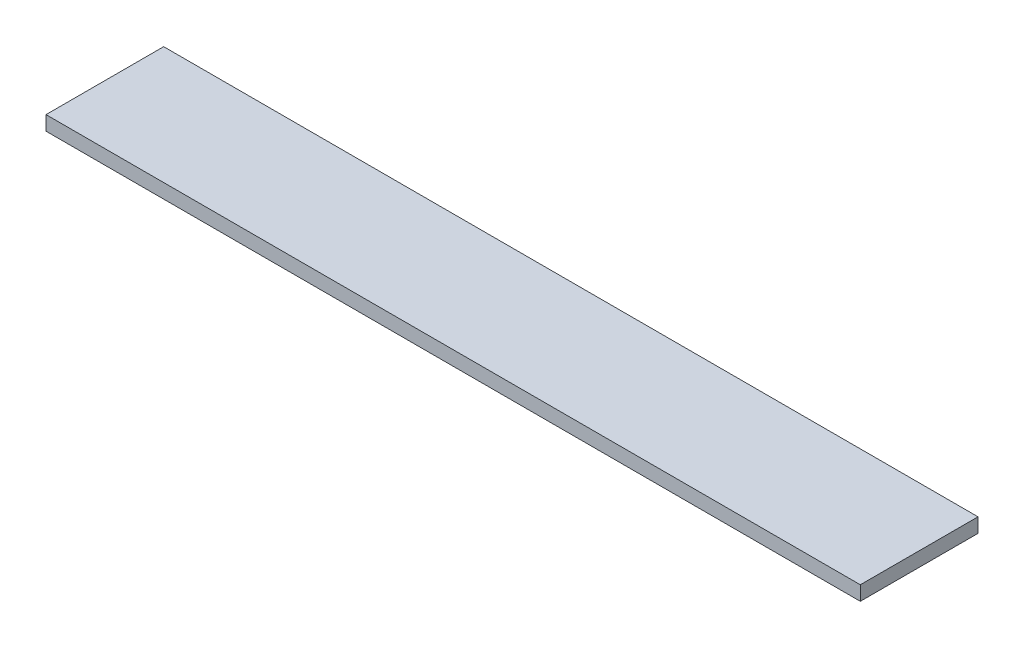
SolidWorks part; units mm, degrees
ref_plane "前视基准面" through (0, 0, 0) normal (0, 0, 1) x (1, 0, 0)
ref_plane "上视基准面" through (0, 0, 0) normal (0, 1, 0) x (1, 0, 0)
ref_plane "右视基准面" through (0, 0, 0) normal (1, 0, 0) x (0, 0, -1)
sketch "草图1" plane through (0, 0, 0) normal (0, 1, 0) x (1, 0, 0)
  line L1 (-1133, -163.75) -> (1133, -163.75)
  line L2 (-1133, -163.75) -> (-1133, 163.75)
  line L3 (-1133, 163.75) -> (1133, 163.75)
  line L4 (1133, -163.75) -> (1133, 163.75)
  line L5 (-1133, -163.75) -> (1133, 163.75) construction
  line L6 (-1133, 163.75) -> (1133, -163.75) construction
  point P0 (0, 0)
  dimension "D1" = 2266
  dimension "D2" = 327.5
extrude "凸台-拉伸1" add sketch "草图1" along normal blind 40
